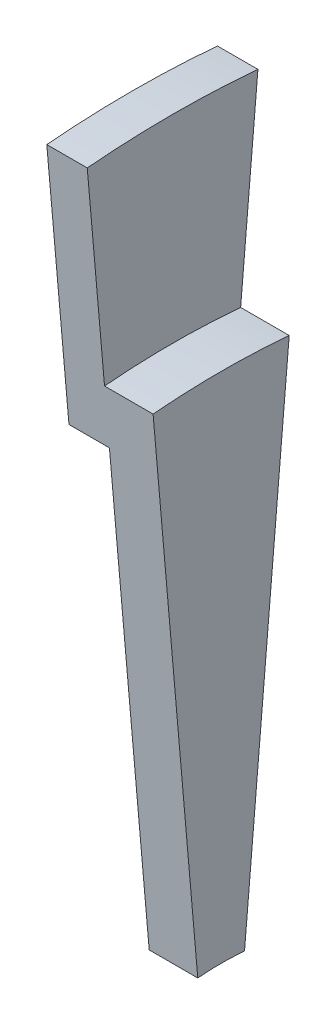
SolidWorks part; units mm, degrees
ref_plane "Front Plane" through (0, 0, 0) normal (0, 0, 1) x (1, 0, 0)
ref_plane "Top Plane" through (0, 0, 0) normal (0, 1, 0) x (1, 0, 0)
ref_plane "Right Plane" through (0, 0, 0) normal (1, 0, 0) x (0, 0, -1)
sketch "Sketch1" plane through (0, 0, 0) normal (0, 0, 1) x (1, 0, 0)
  line L0 (0, 0) -> (-11.5055, 0) construction
  line L1 (-109.9542, 39.4057) -> (-109.9542, 31.426)
  line L2 (-109.9542, 42) -> (-109.9542, -42) construction
  line L3 (-109.9542, 31.426) -> (-109.9542, -31.426) construction
  line L4 (-109.9542, 31.426) -> (-108, 31.426)
  line L5 (-108, 31.426) -> (-108, -31.426) construction
  line L6 (-108, 0) -> (-108, 114) construction
  line L7 (-108, 31.426) -> (-108, 10.7949)
  line L8 (-108, 24.55) -> (-108, -24.55) construction
  line L9 (-108, 10.7949) -> (-109.9542, 10.7949)
  line L10 (-111.5819, 29.1632) -> (-111.5819, 39.4057)
  line L11 (-111.5819, 39.4057) -> (-109.9542, 39.4057)
  line L12 (-111.5819, 29.1632) -> (-109.9542, 29.1632)
  line L13 (-109.9542, 29.1632) -> (-109.9542, 10.7949)
revolve "Revolve1" add sketch "Sketch1" angle 10 mid plane about L0
